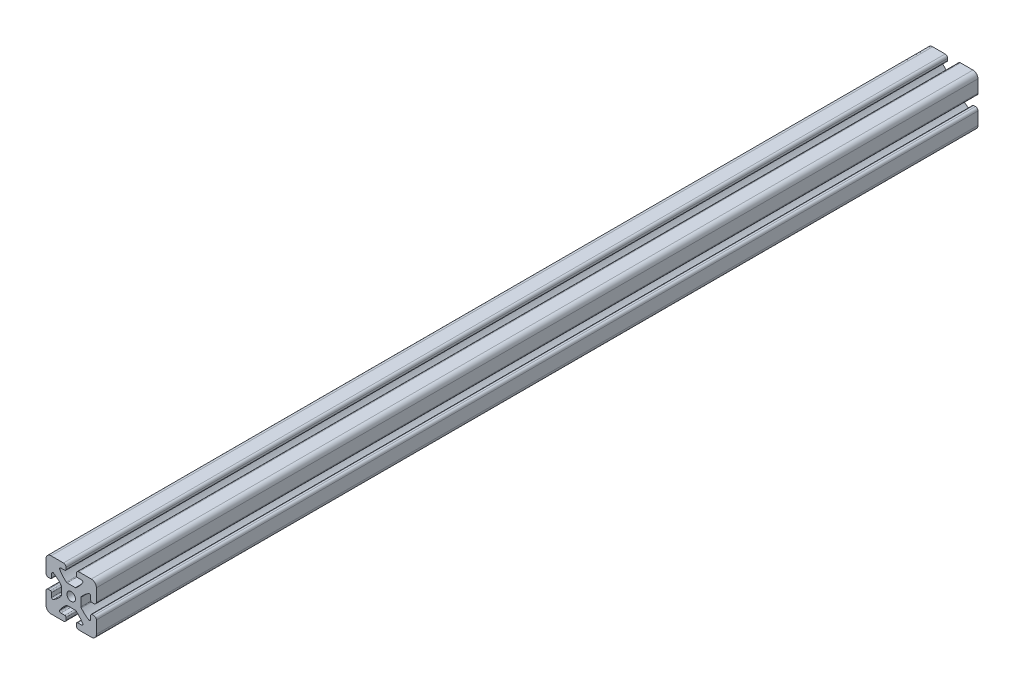
SolidWorks part; units mm, degrees
ref_plane "Front Plane" through (0, 0, 0) normal (0, 0, 1) x (1, 0, 0)
ref_plane "Top Plane" through (0, 0, 0) normal (0, 1, 0) x (1, 0, 0)
ref_plane "Right Plane" through (0, 0, 0) normal (1, 0, 0) x (0, 0, -1)
sketch "Sketch1" plane through (0, 0, 0) normal (0, 0, 1) x (1, 0, 0)
  line L0 (-75.7088, -20.1458) -> (-72.5526, -20.1458)
  line L1 (-70.701, -12.3958) -> (-67.4526, -12.3958)
  line L2 (-96.3499, -4.6458) -> (-39.5519, -4.6458) construction
  line L3 (-87.4526, 11.3542) -> (-87.4526, 1.3542)
  line L4 (-83.4526, -24.6458) -> (-73.5526, -24.6458)
  line L5 (-87.4526, -10.6458) -> (-87.4526, -20.6458)
  line L6 (-83.4526, 15.3542) -> (-73.4526, 15.3542)
  line L7 (-47.4526, -10.6458) -> (-47.4526, -20.6458)
  line L8 (-51.4526, -24.6458) -> (-61.4526, -24.6458)
  line L9 (-59.1964, -20.1458) -> (-62.4526, -20.1458)
  line L10 (-51.4526, 15.3542) -> (-61.4526, 15.3542)
  line L11 (-47.4526, 11.3542) -> (-47.4526, 1.3542)
  line L12 (-64.2043, -12.3958) -> (-67.4526, -12.3958)
  line L13 (-71.5526, -21.1458) -> (-71.5526, -22.6458)
  line L14 (-63.3526, -21.1458) -> (-63.3526, -22.6458)
  line L15 (-50.9526, -8.7458) -> (-49.4526, -8.7458)
  line L16 (-51.9526, -12.902) -> (-51.9526, -9.7458)
  line L17 (-59.7026, -7.8942) -> (-59.7026, -4.6458)
  line L18 (-50.9526, -0.5458) -> (-49.4526, -0.5458)
  line L19 (-51.9526, 3.6104) -> (-51.9526, 0.3542)
  line L20 (-59.7026, -1.3975) -> (-59.7026, -4.6458)
  line L21 (-63.3526, 11.8542) -> (-63.3526, 13.3542)
  line L22 (-59.1964, 10.8542) -> (-62.3526, 10.8542)
  line L23 (-63.8526, 3.1042) -> (-67.4526, 3.1042)
  line L24 (-71.5526, 11.8542) -> (-71.5526, 13.3542)
  line L25 (-75.7088, 10.8542) -> (-72.4526, 10.8542)
  line L26 (-71.0526, 3.1042) -> (-67.4526, 3.1042)
  line L27 (-83.9526, -0.5458) -> (-85.4526, -0.5458)
  line L28 (-82.9526, 3.6104) -> (-82.9526, 0.4542)
  line L29 (-75.2026, -1.3975) -> (-75.2026, -4.6458)
  line L30 (-83.9526, -8.7458) -> (-85.4526, -8.7458)
  line L31 (-82.9526, -12.902) -> (-82.9526, -9.6458)
  line L32 (-75.2026, -7.8942) -> (-75.2026, -4.6458)
  line L33 (-67.4526, 16.4313) -> (-67.4526, -26.9314) construction
  arc A0 (-71.3325, -12.6205) -> (-76.5532, -18.6101) centre (-55.648, -31.5616) ccw
  arc A1 (-76.5532, -18.6101) -> (-75.7088, -20.1458) centre (-75.7088, -19.1458) ccw
  arc A2 (-70.701, -12.3958) -> (-71.3325, -12.6205) centre (-70.701, -13.3958) ccw
  arc A3 (-83.4526, 15.3542) -> (-87.4526, 11.3542) centre (-83.4526, 11.3542) ccw
  arc A4 (-87.4526, -20.6458) -> (-83.4526, -24.6458) centre (-83.4526, -20.6458) ccw
  arc A6 (-63.5727, -12.6205) -> (-64.2043, -12.3958) centre (-64.2043, -13.3958) ccw
  arc A7 (-58.352, -18.6101) -> (-63.5727, -12.6205) centre (-79.2572, -31.5616) ccw
  arc A8 (-59.1964, -20.1458) -> (-58.352, -18.6101) centre (-59.1964, -19.1458) ccw
  arc A9 (-51.4526, -24.6458) -> (-47.4526, -20.6458) centre (-51.4526, -20.6458) ccw
  arc A10 (-47.4526, 11.3542) -> (-51.4526, 15.3542) centre (-51.4526, 11.3542) ccw
  circle A11 centre (-67.4526, -4.6458) radius 3.4
  arc A12 (-71.5526, -21.1458) -> (-72.5526, -20.1458) centre (-72.5526, -21.1458) ccw
  arc A13 (-73.5526, -24.6458) -> (-71.5526, -22.6458) centre (-73.5526, -22.6458) ccw
  arc A14 (-62.3526, -20.1458) -> (-63.3526, -21.1458) centre (-62.3526, -21.1458) ccw
  arc A15 (-63.3526, -22.6458) -> (-61.3526, -24.6458) centre (-61.3526, -22.6458) ccw
  arc A16 (-59.7026, -7.8942) -> (-59.478, -8.5257) centre (-58.7026, -7.8942) ccw
  arc A17 (-59.478, -8.5257) -> (-53.4884, -13.7464) centre (-40.5368, 7.1588) ccw
  arc A18 (-53.4884, -13.7464) -> (-51.9526, -12.902) centre (-52.9526, -12.902) ccw
  arc A19 (-50.9526, -8.7458) -> (-51.9526, -9.7458) centre (-50.9526, -9.7458) ccw
  arc A20 (-47.4526, -10.7458) -> (-49.4526, -8.7458) centre (-49.4526, -10.7458) ccw
  arc A21 (-59.478, -0.7659) -> (-59.7026, -1.3975) centre (-58.7026, -1.3975) ccw
  arc A22 (-53.4884, 4.4548) -> (-59.478, -0.7659) centre (-40.5368, -16.4504) ccw
  arc A23 (-51.9526, 0.4542) -> (-50.9526, -0.5458) centre (-50.9526, 0.4542) ccw
  arc A24 (-49.4526, -0.5458) -> (-47.4526, 1.4542) centre (-49.4526, 1.4542) ccw
  arc A25 (-51.9526, 3.6104) -> (-53.4884, 4.4548) centre (-52.9526, 3.6104) ccw
  arc A26 (-64.2043, 3.1042) -> (-63.5727, 3.3289) centre (-64.2043, 4.1042) ccw
  arc A27 (-63.5727, 3.3289) -> (-58.352, 9.3184) centre (-79.2572, 22.27) ccw
  arc A28 (-58.352, 9.3184) -> (-59.1964, 10.8542) centre (-59.1964, 9.8542) ccw
  arc A29 (-63.3526, 11.8542) -> (-62.3526, 10.8542) centre (-62.3526, 11.8542) ccw
  arc A30 (-61.3526, 15.3542) -> (-63.3526, 13.3542) centre (-61.3526, 13.3542) ccw
  arc A31 (-71.3325, 3.3289) -> (-70.701, 3.1042) centre (-70.701, 4.1042) ccw
  arc A32 (-76.5532, 9.3184) -> (-71.3325, 3.3289) centre (-55.648, 22.27) ccw
  arc A33 (-72.5526, 10.8542) -> (-71.5526, 11.8542) centre (-72.5526, 11.8542) ccw
  arc A34 (-71.5526, 13.3542) -> (-73.5526, 15.3542) centre (-73.5526, 13.3542) ccw
  arc A35 (-75.7088, 10.8542) -> (-76.5532, 9.3184) centre (-75.7088, 9.8542) ccw
  arc A36 (-75.2026, -1.3975) -> (-75.4273, -0.7659) centre (-76.2026, -1.3975) ccw
  arc A37 (-75.4273, -0.7659) -> (-81.4169, 4.4548) centre (-94.3684, -16.4504) ccw
  arc A38 (-81.4169, 4.4548) -> (-82.9526, 3.6104) centre (-81.9526, 3.6104) ccw
  arc A39 (-83.9526, -0.5458) -> (-82.9526, 0.4542) centre (-83.9526, 0.4542) ccw
  arc A40 (-87.4526, 1.4542) -> (-85.4526, -0.5458) centre (-85.4526, 1.4542) ccw
  arc A41 (-75.4273, -8.5257) -> (-75.2026, -7.8942) centre (-76.2026, -7.8942) ccw
  arc A42 (-81.4169, -13.7464) -> (-75.4273, -8.5257) centre (-94.3684, 7.1588) ccw
  arc A43 (-82.9526, -9.7458) -> (-83.9526, -8.7458) centre (-83.9526, -9.7458) ccw
  arc A44 (-85.4526, -8.7458) -> (-87.4526, -10.7458) centre (-85.4526, -10.7458) ccw
  arc A45 (-82.9526, -12.902) -> (-81.4169, -13.7464) centre (-81.9526, -12.902) ccw
extrude "Boss-Extrude1" add sketch "Sketch1" along normal blind 700 contours A45 L31 A43 L30 A44 L5 A4 L4 A13 L13 A12 L0 A1 A0 A2 L1 L12 A6 A7 A8 L9 A14 L14 A15 L8 A9 L7 A20 L15 A19 L16 A18 A17 A16 L17 L20 A21 A22 A25 L19 A23 L18 A24 L11 A10 L10 A30 L21 A29 L22 A28
